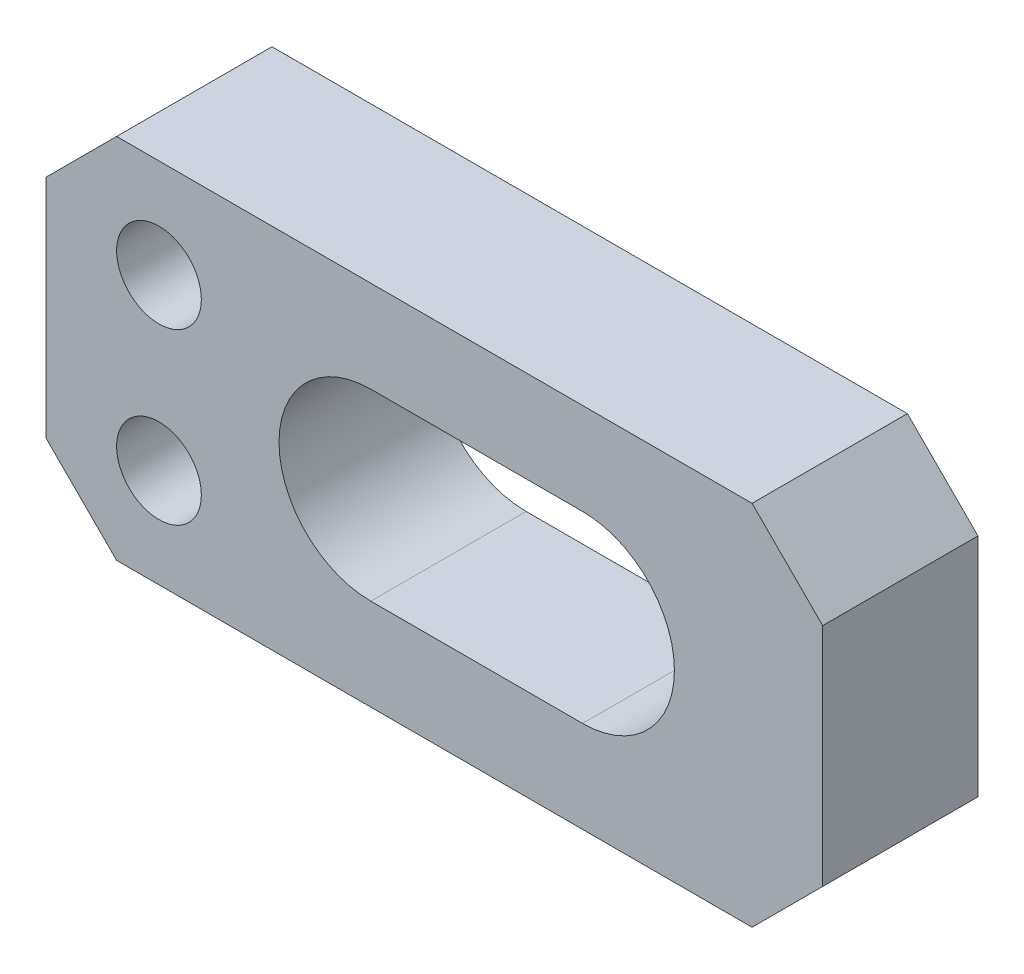
SolidWorks part; units mm, degrees
ref_plane "前视基准面" through (0, 0, 0) normal (0, 0, 1) x (1, 0, 0)
ref_plane "上视基准面" through (0, 0, 0) normal (0, 1, 0) x (1, 0, 0)
ref_plane "右视基准面" through (0, 0, 0) normal (1, 0, 0) x (0, 0, -1)
sketch "草图1" plane through (0, 0, 0) normal (0, 0, 1) x (1, 0, 0)
  line L0 (-4.5, 0) -> (10.5, 0) construction
  line L1 (-27.5, -13) -> (27.5, -13)
  line L2 (-27.5, -13) -> (-27.5, 13)
  line L3 (-27.5, 13) -> (27.5, 13)
  line L4 (27.5, -13) -> (27.5, 13)
  line L5 (-27.5, -13) -> (27.5, 13) construction
  line L6 (-27.5, 13) -> (27.5, -13) construction
  line L7 (-4.5, 6.5) -> (10.5, 6.5)
  line L8 (-4.5, -6.5) -> (10.5, -6.5)
  circle A0 centre (-19.5, 6) radius 3
  circle A1 centre (-19.5, -6) radius 3
  arc A2 (-4.5, 6.5) -> (-4.5, -6.5) centre (-4.5, 0) ccw
  arc A3 (10.5, -6.5) -> (10.5, 6.5) centre (10.5, 0) ccw
  point P0 (0, 0)
  point P11 (3, 0)
  dimension "D1" = 6
  dimension "D5" = 6.5
  dimension "D2" = 8
  dimension "D3" = 7
  dimension "D4" = 7
  dimension "D6" = 23
  dimension "D7" = 15
  dimension "D8" = 26
  dimension "D9" = 17
extrude "凸台-拉伸1" add sketch "草图1" along normal blind 11
chamfer "倒角1" distance 5 angle 45 4 edges at (27.5, -13, 5.5) (27.5, 13, 5.5) (-27.5, -13, 5.5) (-27.5, 13, 5.5)
